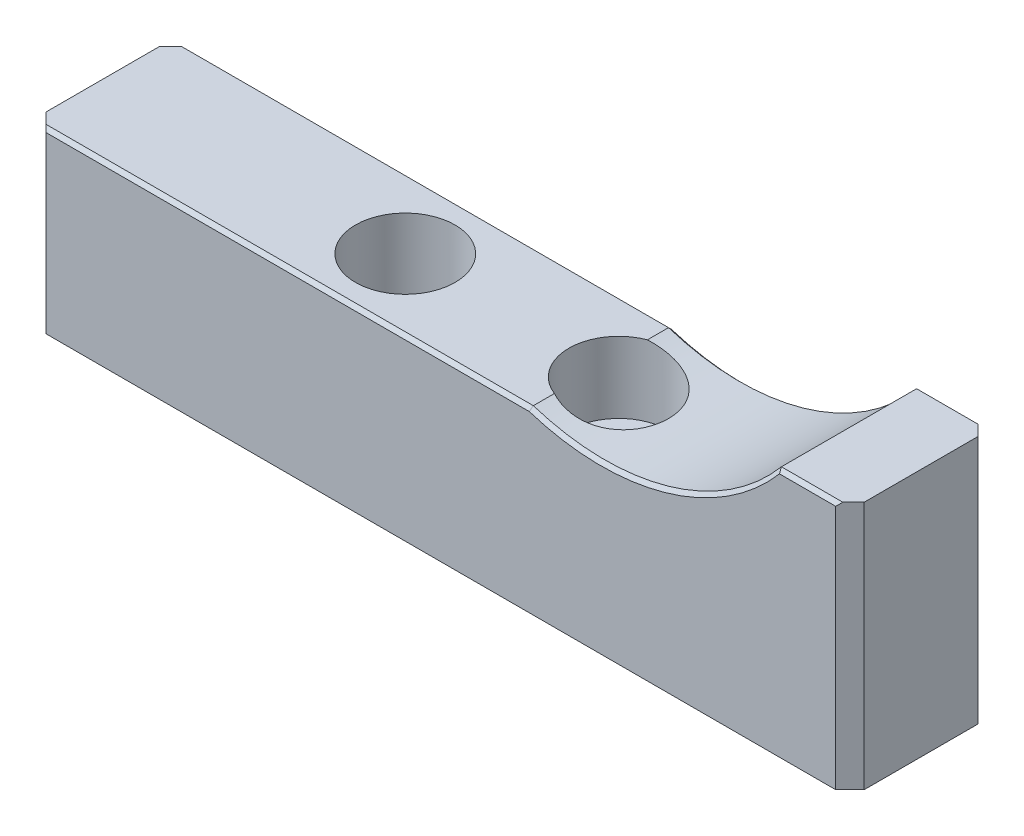
SolidWorks part; units mm, degrees
ref_plane "前视基准面" through (0, 0, 0) normal (0, 0, 1) x (1, 0, 0)
ref_plane "上视基准面" through (0, 0, 0) normal (0, 1, 0) x (1, 0, 0)
ref_plane "右视基准面" through (0, 0, 0) normal (1, 0, 0) x (0, 0, -1)
sketch "草图2" plane through (0, 0, 0) normal (0, 0, 1) x (1, 0, 0)
  line L0 (0, 0) -> (0, 25)
  line L1 (0, 25) -> (70, 25)
  line L2 (104.869, 35) -> (115, 35)
  line L3 (115, 35) -> (115, 0)
  line L4 (115, 0) -> (0, 0)
  arc A0 (70, 25) -> (104.869, 35) centre (80, 55.9233) ccw
  dimension "D3" = 32.5
  dimension "D1" = 25
  dimension "D2" = 35
  dimension "D4" = 115
  dimension "D5" = 80
  dimension "D6" = 70
extrude "凸台-拉伸1" add sketch "草图2" along normal blind 20
sketch "草图4" plane through (0, 35, 0) normal (0, 1, 0) x (1, 0, 0)
  line L0 (115, -10) -> (0, -10) construction
  line L1 (115, -20) -> (115, 0) construction
  line L2 (57.5, -10) -> (57.5, 26.5001) construction
  circle A0 centre (42.5, -10) radius 7
  circle A1 centre (72.5, -10) radius 7
  dimension "D1" = 14
  dimension "D3" = 30
  dimension "D2" = 115
extrude "切除-拉伸1" cut sketch "草图4" against normal blind 20
sketch "草图5" plane through (0, 15, 0) normal (0, 1, 0) x (1, 0, 0)
  circle A0 centre (42.5, -10) radius 4.5
  circle A1 centre (72.5, -10) radius 4.5
  dimension "D1" = 9
extrude "切除-拉伸2" cut sketch "草图5" against normal blind 20
chamfer "倒角1" distance 2 angle 45 4 edges at (0, 12.5, 20) (0, 12.5, 0) (115, 17.5, 0) (115, 17.5, 20)
chamfer "倒角2" distance 0.5 angle 45 6 edges at (108.9345, 35, 0) (88.9594, 24.6826, 0) (36, 25, 0) (108.9345, 35, 20) (88.9594, 24.6826, 20) (36, 25, 20)
